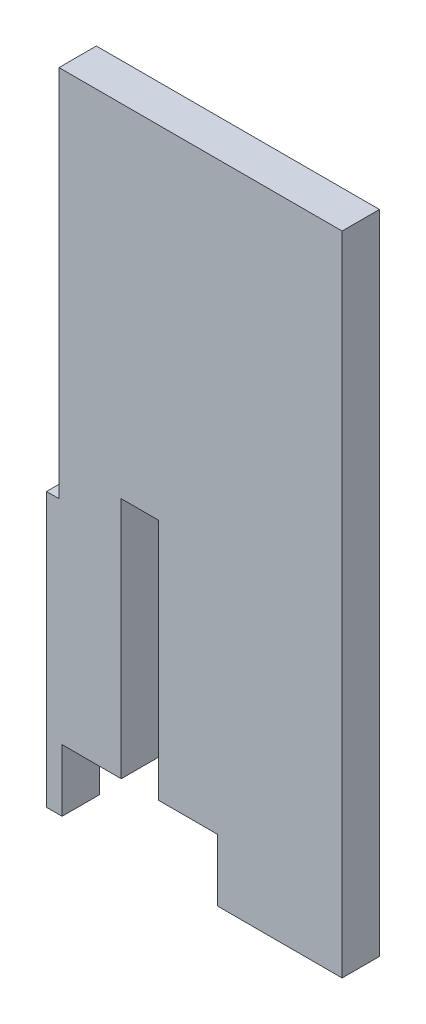
SolidWorks part; units mm, degrees
material "Q235B"
ref_plane "Front Plane" through (0, 0, 0) normal (0, 0, 1) x (1, 0, 0)
ref_plane "Top Plane" through (0, 0, 0) normal (0, 1, 0) x (1, 0, 0)
ref_plane "Right Plane" through (0, 0, 0) normal (1, 0, 0) x (0, 0, -1)
sketch "Sketch1" plane through (0, 0, 0) normal (0, 0, 1) x (1, 0, 0)
  line L0 (127.0206, -33.4453) -> (107.0206, -33.4453)
  line L2 (107.0206, -33.4453) -> (107.0206, 70.5147)
  line L4 (127.0206, -33.4453) -> (127.0206, -23.4651)
  line L6 (152.0224, -33.4453) -> (172.0224, -33.4453)
  line L7 (172.0224, -33.4453) -> (172.0224, 70.5147)
  line L8 (172.0224, 70.5147) -> (107.0206, 70.5147)
  line L9 (127.0206, -23.4651) -> (152.0224, -23.4651)
  line L10 (152.0224, -23.4651) -> (152.0224, -33.4453)
  dimension "D1" = 20
  dimension "D2" = 25.0018
  dimension "D3" = 20
  dimension "D4" = 103.96
  dimension "D5" = 9.9802
extrude "Boss-Extrude1" add sketch "Sketch1" along normal blind 6
sketch "Sketch3" plane through (0, 0, 0) normal (0, 0, -1) x (-1, 0, 0)
  line L0 (-142.5224, 15.5147) -> (-142.5224, -44.4853)
  line L1 (-142.5224, 15.5147) -> (-136.5224, 15.5147)
  line L2 (-136.5224, 15.5147) -> (-136.5224, -44.4853)
  line L3 (-142.5224, -44.4853) -> (-136.5224, -44.4853)
  line L4 (-152.0224, -23.4651) -> (-152.0224, -33.4453) construction
  line L5 (-172.0224, 70.5147) -> (-107.0206, 70.5147) construction
  point P2 (-139.5224, -44.4853)
  dimension "D2" = 12.5
  dimension "D3" = 55
  dimension "D4" = 60
  dimension "D1" = 6
extrude "Cut-Extrude1" cut sketch "Sketch3" against normal blind 10
sketch "Sketch4" plane through (0, 0, 6) normal (0, 0, 1) x (1, 0, 0)
  line L1 (124.5224, -36.5804) -> (107.0206, -36.5804)
  line L2 (107.0206, 70.5147) -> (107.0206, -33.4453) construction
  line L3 (107.0206, -36.5804) -> (107.0206, 70.5147)
  line L4 (107.0206, 70.5147) -> (120.5125, 70.5147)
  line L5 (172.0224, 70.5147) -> (107.0206, 70.5147) construction
  line L6 (124.5224, 10.5147) -> (124.5224, -36.5804)
  line L7 (124.5224, 10.5147) -> (126.5224, 10.5147)
  line L8 (126.5224, 10.5147) -> (126.5224, 70.5147)
  line L9 (172.0224, 70.5147) -> (107.0206, 70.5147) construction
  line L10 (126.5224, 70.5147) -> (120.5125, 70.5147)
  dimension "D2" = 2
  dimension "D3" = 60
extrude "Cut-Extrude2" cut sketch "Sketch4" against normal through all
